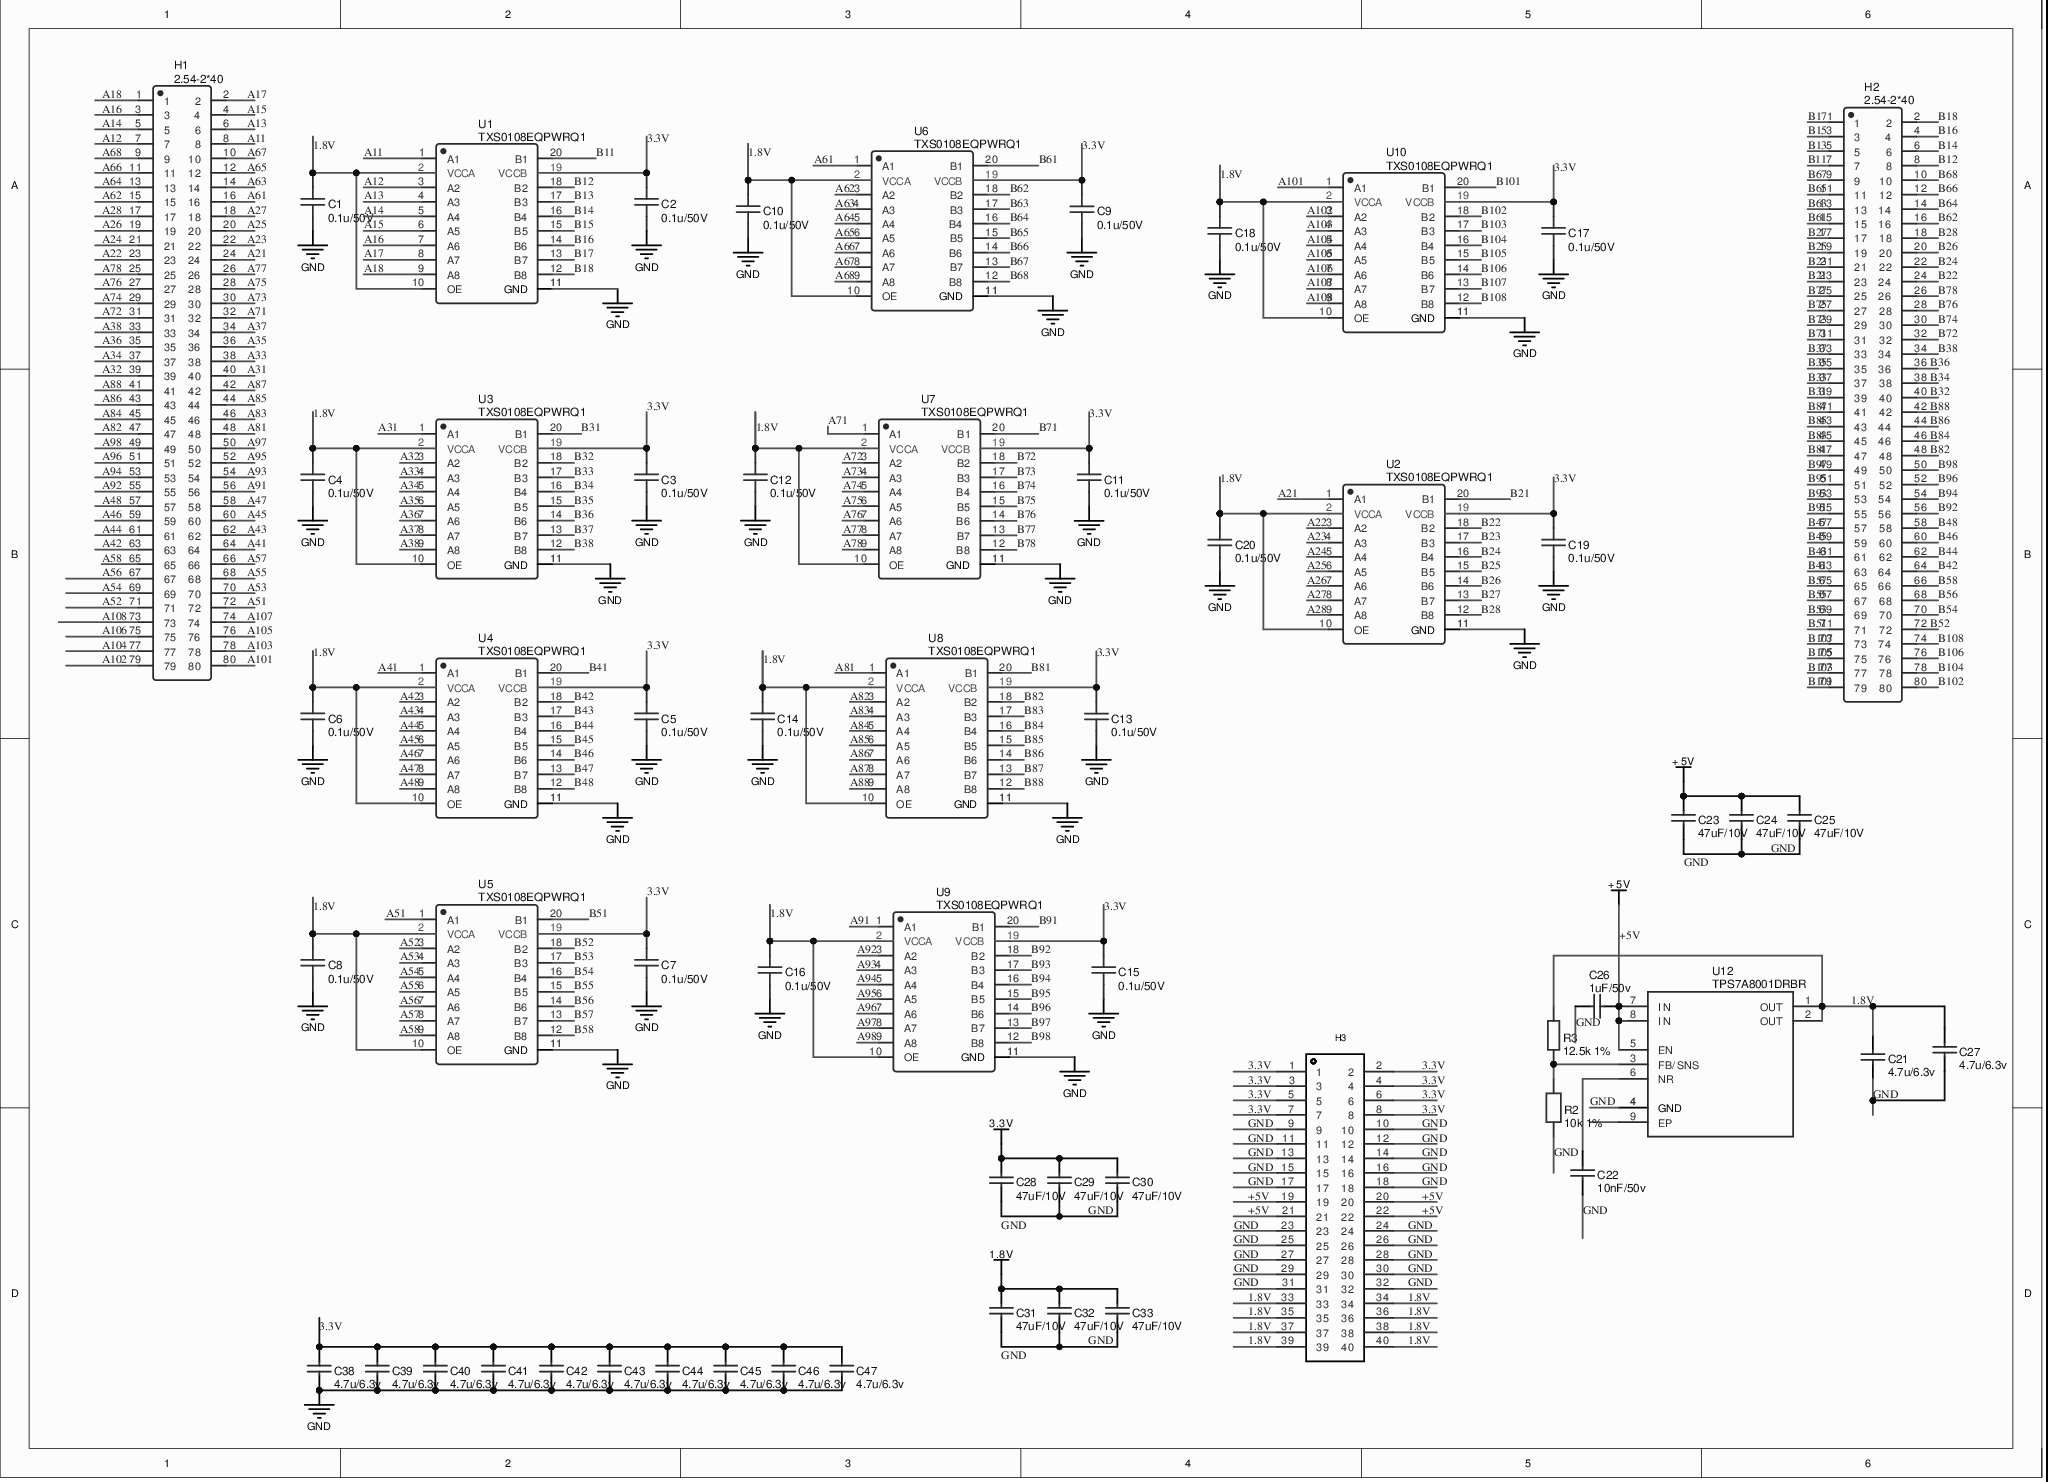
[diagram p0: MISC79033-8.schdoc]
# Altium project MISC79033-2.PrjPCB
1 sheet, 59 parts. Net scope: global (net labels, ports and power ports of the same name join across sheets).
Board file: MISC79033.pcbdoc

## Sheet MISC79033-8.schdoc
size 357 x 258 mm

### Parts
C1  0.1u/50V  [C0603]
C2  0.1u/50V  [C0603]
C3  0.1u/50V  [C0603]
C4  0.1u/50V  [C0603]
C5  0.1u/50V  [C0603]
C6  0.1u/50V  [C0603]
C7  0.1u/50V  [C0603]
C8  0.1u/50V  [C0603]
C9  0.1u/50V  [C0603]
C10  0.1u/50V  [C0603]
C11  0.1u/50V  [C0603]
C12  0.1u/50V  [C0603]
C13  0.1u/50V  [C0603]
C14  0.1u/50V  [C0603]
C15  0.1u/50V  [C0603]
C16  0.1u/50V  [C0603]
C17  0.1u/50V  [C0603]
C18  0.1u/50V  [C0603]
C19  0.1u/50V  [C0603]
C20  0.1u/50V  [C0603]
C21  4.7u/6.3v  [C0603]
C22  10nF/50v  [C0603]
C23  47uF/10V  [C1206]
C24  47uF/10V  [C1206]
C25  47uF/10V  [C1206]
C26  1uF/50v  [C0603]
C27  4.7u/6.3v  [C0603]
C28  47uF/10V  [C1206]
C29  47uF/10V  [C1206]
C30  47uF/10V  [C1206]
C31  47uF/10V  [C1206]
C32  47uF/10V  [C1206]
C33  47uF/10V  [C1206]
C38  4.7u/6.3v  [C0603]
C39  4.7u/6.3v  [C0603]
C40  4.7u/6.3v  [C0603]
C41  4.7u/6.3v  [C0603]
C42  4.7u/6.3v  [C0603]
C43  4.7u/6.3v  [C0603]
C44  4.7u/6.3v  [C0603]
C45  4.7u/6.3v  [C0603]
C46  4.7u/6.3v  [C0603]
C47  4.7u/6.3v  [C0603]
H1  2.54-2*40  [HDR-TH_80P-P2.54-V-M-R2-C40-S2.54]
H2  2.54-2*40  [HDR-TH_80P-P2.54-V-M-R2-C40-S2.54]
H3  B-2100S40P-B110  [HDR-TH_40P-P2.54-V-M-R2-C20-S2.54]  (value not drawn)
R2  10k 1%  [R0603]
R3  12.5k 1%  [R0603]
U1  TXS0108EQPWRQ1  [TSSOP-20_L6.5-W4.4-P0.65-LS6.4-BL]
U2  TXS0108EQPWRQ1  [TSSOP-20_L6.5-W4.4-P0.65-LS6.4-BL]
U3  TXS0108EQPWRQ1  [TSSOP-20_L6.5-W4.4-P0.65-LS6.4-BL]
U4  TXS0108EQPWRQ1  [TSSOP-20_L6.5-W4.4-P0.65-LS6.4-BL]
U5  TXS0108EQPWRQ1  [TSSOP-20_L6.5-W4.4-P0.65-LS6.4-BL]
U6  TXS0108EQPWRQ1  [TSSOP-20_L6.5-W4.4-P0.65-LS6.4-BL]
U7  TXS0108EQPWRQ1  [TSSOP-20_L6.5-W4.4-P0.65-LS6.4-BL]
U8  TXS0108EQPWRQ1  [TSSOP-20_L6.5-W4.4-P0.65-LS6.4-BL]
U9  TXS0108EQPWRQ1  [TSSOP-20_L6.5-W4.4-P0.65-LS6.4-BL]
U10  TXS0108EQPWRQ1  [TSSOP-20_L6.5-W4.4-P0.65-LS6.4-BL]
U12  TPS7A8001DRBR  [VSON-8_L3.0-W3.0-P0.65-TL-EP]

### Nets
1.8V: C1.2 C4.2 C6.2 C8.2 C10.2 C12.2 C14.2 C16.2 C18.2 C20.2 C21.2 C27.2 C31.2 C32.2 C33.2 H3.33 H3.34 H3.35 H3.36 H3.37 H3.38 H3.39 H3.40 R3.1 U1.2(VCCA) U1.10(OE) U2.2(VCCA) U2.10(OE) U3.2(VCCA) U3.10(OE) U4.2(VCCA) U4.10(OE) U5.2(VCCA) U5.10(OE) U6.2(VCCA) U6.10(OE) U7.2(VCCA) U7.10(OE) U8.2(VCCA) U8.10(OE) U9.2(VCCA) U9.10(OE) U10.2(VCCA) U10.10(OE) U12.1(OUT) U12.2(OUT)
3.3V: C2.2 C3.2 C5.2 C7.2 C9.2 C11.2 C13.2 C15.2 C17.2 C19.2 C28.2 C29.2 C30.2 C38.2 C39.2 C40.2 C41.2 C42.2 C43.2 C44.2 C45.2 C46.2 C47.2 H3.1 H3.2 H3.3 H3.4 H3.5 H3.6 H3.7 H3.8 U1.19(VCCB) U2.19(VCCB) U3.19(VCCB) U4.19(VCCB) U5.19(VCCB) U6.19(VCCB) U7.19(VCCB) U8.19(VCCB) U9.19(VCCB) U10.19(VCCB)
+5V: C23.2 C24.2 C25.2 C26.1 H3.19 H3.20 H3.21 H3.22 U12.5(EN) U12.7(IN) U12.8(IN)
GND: C1.1 C2.1 C3.1 C4.1 C5.1 C6.1 C7.1 C8.1 C9.1 C10.1 C11.1 C12.1 C13.1 C14.1 C15.1 C16.1 C17.1 C18.1 C19.1 C20.1 C21.1 C22.1 C23.1 C24.1 C25.1 C26.2 C27.1 C28.1 C29.1 C30.1 C31.1 C32.1 C33.1 C38.1 C39.1 C40.1 C41.1 C42.1 C43.1 C44.1 C45.1 C46.1 C47.1 H3.9 H3.10 H3.11 H3.12 H3.13 H3.14 H3.15 H3.16 H3.17 H3.18 H3.23 H3.24 H3.25 H3.26 H3.27 H3.28 H3.29 H3.30 H3.31 H3.32 R2.1 U1.11(GND) U2.11(GND) U3.11(GND) U4.11(GND) U5.11(GND) U6.11(GND) U7.11(GND) U8.11(GND) U9.11(GND) U10.11(GND) U12.4(GND)
A11: H1.8 U1.1(A1)
A12: H1.7 U1.3(A2)
A13: H1.6 U1.4(A3)
A14: H1.5 U1.5(A4)
A15: H1.4 U1.6(A5)
A16: H1.3 U1.7(A6)
A17: H1.2 U1.8(A7)
A18: H1.1 U1.9(A8)
A21: H1.24 U2.1(A1)
A22: H1.23 U2.3(A2)
A23: H1.22 U2.4(A3)
A24: H1.21 U2.5(A4)
A25: H1.20 U2.6(A5)
A26: H1.19 U2.7(A6)
A27: H1.18 U2.8(A7)
A28: H1.17 U2.9(A8)
A31: H1.40 U3.1(A1)
A32: H1.39 U3.3(A2)
A33: H1.38 U3.4(A3)
A34: H1.37 U3.5(A4)
A35: H1.36 U3.6(A5)
A36: H1.35 U3.7(A6)
A37: H1.34 U3.8(A7)
A38: H1.33 U3.9(A8)
A41: H1.64 U4.1(A1)
A42: H1.63 U4.3(A2)
A43: H1.62 U4.4(A3)
A44: H1.61 U4.5(A4)
A45: H1.60 U4.6(A5)
A46: H1.59 U4.7(A6)
A47: H1.58 U4.8(A7)
A48: H1.57 U4.9(A8)
A51: H1.72 U5.1(A1)
A52: H1.71 U5.3(A2)
A53: H1.70 U5.4(A3)
A54: H1.69 U5.5(A4)
A55: H1.68 U5.6(A5)
A56: H1.67 U5.7(A6)
A57: H1.66 U5.8(A7)
A58: H1.65 U5.9(A8)
A61: H1.16 U6.1(A1)
A62: H1.15 U6.3(A2)
A63: H1.14 U6.4(A3)
A64: H1.13 U6.5(A4)
A65: H1.12 U6.6(A5)
A66: H1.11 U6.7(A6)
A67: H1.10 U6.8(A7)
A68: H1.9 U6.9(A8)
A71: H1.32 U7.1(A1)
A72: H1.31 U7.3(A2)
A73: H1.30 U7.4(A3)
A74: H1.29 U7.5(A4)
A75: H1.28 U7.6(A5)
A76: H1.27 U7.7(A6)
A77: H1.26 U7.8(A7)
A78: H1.25 U7.9(A8)
A81: H1.48 U8.1(A1)
A82: H1.47 U8.3(A2)
A83: H1.46 U8.4(A3)
A84: H1.45 U8.5(A4)
A85: H1.44 U8.6(A5)
A86: H1.43 U8.7(A6)
A87: H1.42 U8.8(A7)
A88: H1.41 U8.9(A8)
A91: H1.56 U9.1(A1)
A92: H1.55 U9.3(A2)
A93: H1.54 U9.4(A3)
A94: H1.53 U9.5(A4)
A95: H1.52 U9.6(A5)
A96: H1.51 U9.7(A6)
A97: H1.50 U9.8(A7)
A98: H1.49 U9.9(A8)
A101: H1.80 U10.1(A1)
A102: H1.79 U10.3(A2)
A103: H1.78 U10.4(A3)
A104: H1.77 U10.5(A4)
A105: H1.76 U10.6(A5)
A106: H1.75 U10.7(A6)
A107: H1.74 U10.8(A7)
A108: H1.73 U10.9(A8)
B11: H2.7 U1.20(B1)
B12: H2.8 U1.18(B2)
B13: H2.5 U1.17(B3)
B14: H2.6 U1.16(B4)
B15: H2.3 U1.15(B5)
B16: H2.4 U1.14(B6)
B17: H2.1 U1.13(B7)
B18: H2.2 U1.12(B8)
B21: H2.23 U2.20(B1)
B22: H2.24 U2.18(B2)
B23: H2.21 U2.17(B3)
B24: H2.22 U2.16(B4)
B25: H2.19 U2.15(B5)
B26: H2.20 U2.14(B6)
B27: H2.17 U2.13(B7)
B28: H2.18 U2.12(B8)
B31: H2.39 U3.20(B1)
B32: H2.40 U3.18(B2)
B33: H2.37 U3.17(B3)
B34: H2.38 U3.16(B4)
B35: H2.35 U3.15(B5)
B36: H2.36 U3.14(B6)
B37: H2.33 U3.13(B7)
B38: H2.34 U3.12(B8)
B41: H2.63 U4.20(B1)
B42: H2.64 U4.18(B2)
B43: H2.61 U4.17(B3)
B44: H2.62 U4.16(B4)
B45: H2.59 U4.15(B5)
B46: H2.60 U4.14(B6)
B47: H2.57 U4.13(B7)
B48: H2.58 U4.12(B8)
B51: H2.71 U5.20(B1)
B52: H2.72 U5.18(B2)
B53: H2.69 U5.17(B3)
B54: H2.70 U5.16(B4)
B55: H2.67 U5.15(B5)
B56: H2.68 U5.14(B6)
B57: H2.65 U5.13(B7)
B58: H2.66 U5.12(B8)
B61: H2.15 U6.20(B1)
B62: H2.16 U6.18(B2)
B63: H2.13 U6.17(B3)
B64: H2.14 U6.16(B4)
B65: H2.11 U6.15(B5)
B66: H2.12 U6.14(B6)
B67: H2.9 U6.13(B7)
B68: H2.10 U6.12(B8)
B71: H2.31 U7.20(B1)
B72: H2.32 U7.18(B2)
B73: H2.29 U7.17(B3)
B74: H2.30 U7.16(B4)
B75: H2.27 U7.15(B5)
B76: H2.28 U7.14(B6)
B77: H2.25 U7.13(B7)
B78: H2.26 U7.12(B8)
B81: H2.47 U8.20(B1)
B82: H2.48 U8.18(B2)
B83: H2.45 U8.17(B3)
B84: H2.46 U8.16(B4)
B85: H2.43 U8.15(B5)
B86: H2.44 U8.14(B6)
B87: H2.41 U8.13(B7)
B88: H2.42 U8.12(B8)
B91: H2.55 U9.20(B1)
B92: H2.56 U9.18(B2)
B93: H2.53 U9.17(B3)
B94: H2.54 U9.16(B4)
B95: H2.51 U9.15(B5)
B96: H2.52 U9.14(B6)
B97: H2.49 U9.13(B7)
B98: H2.50 U9.12(B8)
B101: H2.79 U10.20(B1)
B102: H2.80 U10.18(B2)
B103: H2.77 U10.17(B3)
B104: H2.78 U10.16(B4)
B105: H2.75 U10.15(B5)
B106: H2.76 U10.14(B6)
B107: H2.73 U10.13(B7)
B108: H2.74 U10.12(B8)
NetC22_2: C22.2 U12.6(NR)
NetR2_2: R2.2 R3.2 U12.3(FB/SNS)

Not connected (* = marked no-connect by the designer): U12 9(EP)*

### Notes on the sheet
- Labels drawn without touching a wire or pin: GND

### Library data of the parts
C1-C20 = 0.1u: nameAlias: Value(F); Contributor: LCEDA_Lib; spicePre: C; spiceSymbolName: C_0603_US
C21 C27 C38-C47 = 4.7u: Manufacturer Part: CL10A475KO8NNNC; nameAlias: Value; Supplier: LCSC; Supplier Part: C19666; JLCPCB Part Class: Basic Part; spicePre: C; spiceSymbolName: CL10A475KO8NNNC
C22 = 10nF: Manufacturer Part: CC0603KRX7R9BB103; nameAlias: Value; Supplier: LCSC; Supplier Part: C100042; JLCPCB Part Class: Extended Part; spicePre: C; spiceSymbolName: CC0603KRX7R9BB103
C23-C25 C28-C33 = 4.7uF: Manufacturer Part: CL10A475KO8NNNC; nameAlias: Value; Supplier: LCSC; Supplier Part: C19666; JLCPCB Part Class: Basic Part; spicePre: C; spiceSymbolName: CL10A475KO8NNNC
C26 = 1uF: Manufacturer Part: CL10A105KB8NNNC; nameAlias: Value; Supplier: LCSC; Supplier Part: C15849; JLCPCB Part Class: Basic Part; spicePre: C; spiceSymbolName: CL10A105KB8NNNC
H1 H2 = 2.54-2*40: Contributor: lcsc; Supplier: LCSC; Supplier Part: C2977585; Manufacturer Part: 2.54-2*40; JLCPCB Part Class: Extended Part; spicePre: H; spiceSymbolName: 2.54-2*40
H3 = B-2100S40P-B110: Symbol: 210S-2*20P L=11.6MMGold-plated black; Add into BOM: yes; Pitch: 2.54mm; Pin Structure: 2x20P; Name: B-2100S40P-B110; Device: B-2100S40P-B110; Supplier Part: C124383; Manufacturer Part: B-2100S40P-B110; JLCPCB Part Class: Extended Part; Supplier: LCSC; Convert to PCB: yes; Number of Pins: 40; Row Spacing: 2.54mm; Circluar Pins/Square Pins: -; Current Rating (Max): -; Voltage Rating (Max): -; Length of Mating Pin: 6mm; Insulation Height: 2.54mm; Length of End Connection Pin: 3mm; Contact Plating: -
R2 = (no symbol name): Manufacturer Part: ARG05BTC1002; nameAlias: Value; Contributor: LCSC; Supplier: LCSC; Supplier Part: C406725; JLCPCB Part Class: Extended Part; spicePre: R; spiceSymbolName: ARG05BTC1002
R3 = (no symbol name): nameAlias: Value; Contributor: LCSC; Supplier: LCSC; Supplier Part: C337058; JLCPCB Part Class: Extended Part; spicePre: R
U1-U10 = TXS0108EQPWRQ1: Contributor: LCSC; Supplier: LCSC; Supplier Part: C1021790; Manufacturer Part: TXS0108EQPWRQ1; JLCPCB Part Class: Extended Part; spicePre: U; spiceSymbolName: TXS0108EQPWRQ1
U12 = TPS7A8001DRBR: Supplier: LCSC; Manufacturer Part: TPS7A8001DRBR; Supplier Part: C105265; JLCPCB Part Class: Extended Part; spicePre: U; spiceSymbolName: TPS7A8001DRBR